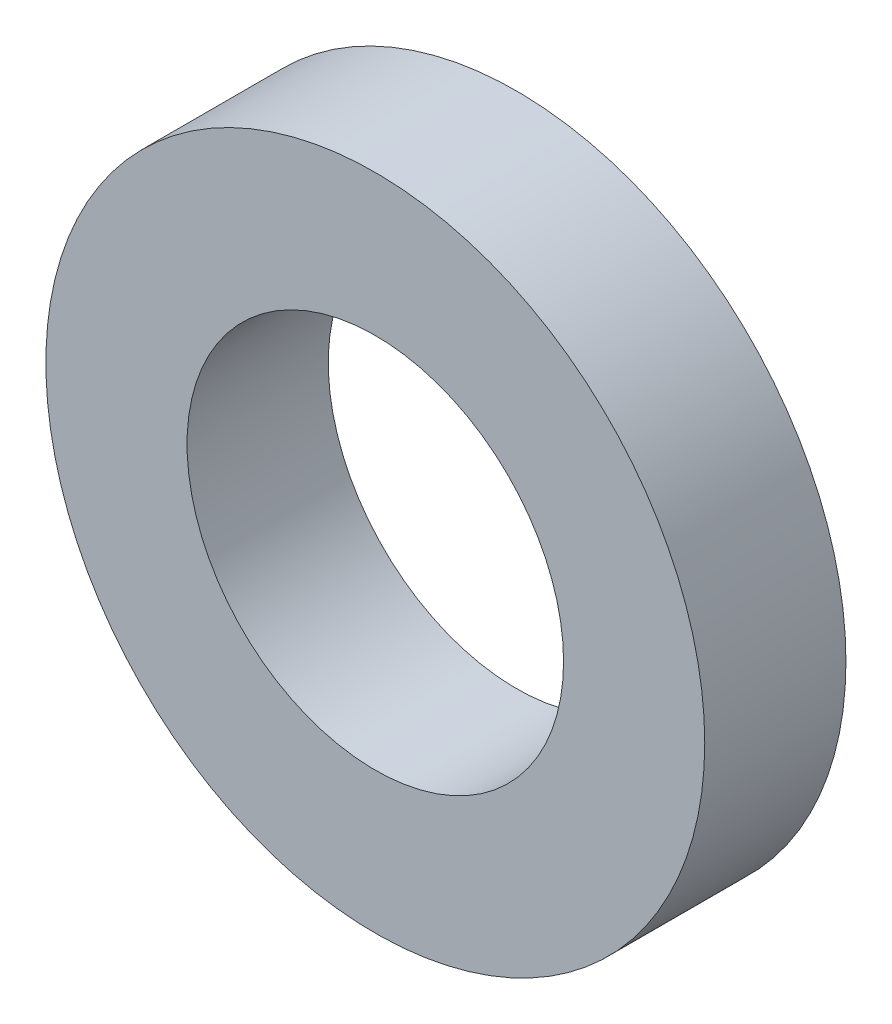
from build123d import *

# Parameters (mm, degrees)
SKETCH1_R           = 35
SKETCH1_R_2         = 20
BOSS_EXTRUDE1_DEPTH = 15


with BuildPart() as part:
    # Sketch1 → Boss-Extrude1 (new body)
    with BuildSketch(Plane.XY):
        Circle(SKETCH1_R)
        Circle(SKETCH1_R_2, mode=Mode.SUBTRACT)
    extrude(amount=BOSS_EXTRUDE1_DEPTH)


solid = part.part
